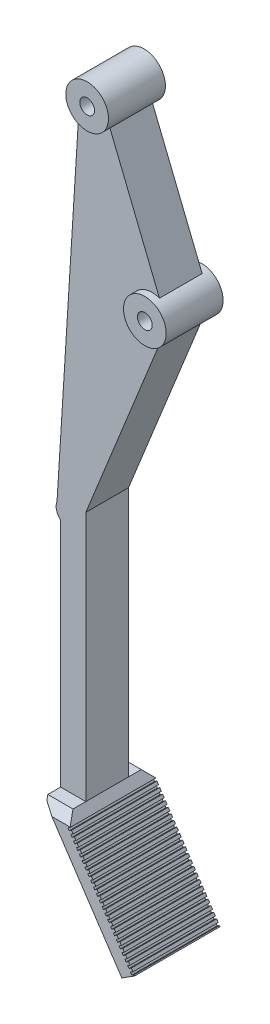
SolidWorks part; units mm, degrees
ref_plane "Front Plane" through (0, 0, 0) normal (0, 0, 1) x (1, 0, 0)
ref_plane "Top Plane" through (0, 0, 0) normal (0, 1, 0) x (1, 0, 0)
ref_plane "Right Plane" through (0, 0, 0) normal (1, 0, 0) x (0, 0, -1)
other "Configuration Table"
sketch "Sketch1" plane through (0, 0, 0) normal (0, 0, 1) x (1, 0, 0)
  circle A0 centre (0, 0) radius 7.5
  dimension "D1" = 15
extrude "Boss-Extrude1" add sketch "Sketch1" along normal mid plane 20
sketch "Sketch2" plane through (0, 0, 0) normal (0, 0, 1) x (1, 0, 0)
  line L0 (0, 0) -> (0, -45.3837) construction
  line L1 (5.5028, -5.096) -> (24.9744, -53.29)
  line L2 (-5.395, -5.2099) -> (15.5663, -57.0911)
  circle A0 centre (0, 0) radius 7.5 construction
  arc A1 (-5.395, -5.2099) -> (5.5028, -5.096) centre (0, 0) ccw
  arc A2 (24.9744, -53.29) -> (15.5663, -57.0911) centre (20.2704, -55.1906) cw
  dimension "D1" = 22
extrude "Boss-Extrude2" add sketch "Sketch2" along normal mid plane 15
sketch "Sketch3" plane through (0, 0, 10) normal (0, 0, 1) x (1, 0, 0)
  circle A0 centre (0, 0) radius 2.6
  dimension "D1" = 5.2
extrude "Cut-Extrude1" cut sketch "Sketch3" against normal through all
sketch "Sketch5" plane through (0, 0, 0) normal (0, 0, 1) x (1, 0, 0)
  line L0 (15.5663, -57.0911) -> (-13.0808, -127.9952)
  line L1 (24.9442, -57.1644) -> (-4.9935, -131.2627)
  line L2 (20.2704, -55.1906) -> (20.2704, -167.243) construction
  arc A0 (15.5663, -57.0911) -> (24.9744, -53.29) centre (20.2704, -55.1906) ccw construction
  arc A1 (15.5663, -57.0911) -> (24.9442, -57.1644) centre (20.2704, -55.1906) ccw
  arc A2 (-13.0808, -127.9952) -> (-4.9935, -131.2627) centre (-9.0371, -129.6289) ccw
  dimension "D1" = 22
  dimension "D2" = 80
extrude "Boss-Extrude3" add sketch "Sketch5" along normal mid plane 15
sketch "Sketch6" plane through (0, 0, 0) normal (0, 0, 1) x (1, 0, 0)
  circle A0 centre (20.2704, -55.1906) radius 7.5
  dimension "D1" = 15
extrude "Boss-Extrude4" add sketch "Sketch6" along normal mid plane 20
sketch "Sketch7" plane through (0, 0, 10) normal (0, 0, 1) x (1, 0, 0)
  circle A0 centre (20.2704, -55.1906) radius 2.6
  dimension "D1" = 5.2
extrude "Cut-Extrude2" cut sketch "Sketch7" against normal through all
sketch "Sketch11" plane through (0, 0, 0) normal (0, 0, 1) x (1, 0, 0)
  line L0 (-5.395, -5.2099) -> (-13.0808, -127.9952)
  line L1 (-5.395, -5.2099) -> (13.4972, -51.9698)
  line L2 (14.4321, -59.8985) -> (-13.0808, -127.9952)
  line L3 (14.4321, -59.8985) -> (-13.0808, -127.9952) construction
  arc A1 (13.4972, -51.9698) -> (14.4321, -59.8985) centre (20.2704, -55.1906) ccw
extrude "Boss-Extrude8" add sketch "Sketch11" along normal mid plane 15
sketch "Sketch16" plane through (0, 0, 0) normal (0, 0, 1) x (1, 0, 0)
  line L0 (-4.9935, -131.2627) -> (22.9045, -62.2128) construction
  line L1 (-11.8087, -126.2616) -> (-2.9729, -126.2616)
  line L2 (-11.8087, -126.2616) -> (-11.8087, -214.2616)
  line L3 (-11.8087, -214.2616) -> (-2.9729, -214.2616)
  line L4 (-2.9729, -126.2616) -> (-2.9729, -214.2616)
  arc A0 (-13.0808, -127.9952) -> (-4.9935, -131.2627) centre (-9.0371, -129.6289) ccw construction
  dimension "D1" = 88
extrude "Boss-Extrude9" add sketch "Sketch16" along normal mid plane 15
sketch "Sketch17" plane through (0, 0, 0) normal (0, 0, -1) x (-1, 0, 0)
  line L3 (11.8087, -214.2616) -> (2.9729, -214.2616)
  line L4 (7.3908, -214.2616) -> (7.3908, -121.3362) construction
  line L5 (-21.6957, -251.2326) -> (2.9729, -214.2616)
  line L6 (-15.4953, -255.1822) -> (-21.6957, -251.2326)
  line L7 (11.8087, -214.2616) -> (-15.4953, -255.1822)
  line L8 (11.8087, -214.2616) -> (2.9729, -214.2616) construction
  line L9 (2.9729, -214.2616) -> (2.9729, -126.2616) construction
  line L10 (11.8087, -132.9962) -> (11.8087, -214.2616) construction
extrude "Boss-Extrude10" add sketch "Sketch17" along normal mid plane 30 contours L3 L5 L6 L7
chamfer "Chamfer1" distance 3 angle 45 2 edges at (-7.3908, -214.2616, 15) (-7.3908, -214.2616, -15)
chamfer "Chamfer2" distance 2 angle 45 2 edges at (2.8442, -236.2219, 15) (2.8442, -236.2219, -15)
sketch "Sketch18" plane through (0, 0, 15) normal (0, 0, 1) x (1, 0, 0)
  line L0 (-0.9223, -217.335) -> (-0.4782, -218.0004)
  line L1 (21.6957, -251.2326) -> (-0.9712, -217.2616) construction
  line L2 (-0.4782, -218.0004) -> (-1.3101, -218.5555)
  line L3 (-1.3101, -218.5555) -> (-1.7541, -217.89)
  line L4 (-1.7541, -217.89) -> (-0.9223, -217.335)
  line L97 (-0.755, -219.3873) -> (0.0768, -218.8323)
  line L98 (0.0768, -218.8323) -> (0.5208, -219.4977)
  line L99 (0.5208, -219.4977) -> (-0.311, -220.0528)
  line L100 (-0.311, -220.0528) -> (-0.755, -219.3873)
  line L101 (0.244, -220.8846) -> (1.0759, -220.3296)
  line L102 (1.0759, -220.3296) -> (1.5199, -220.995)
  line L103 (1.5199, -220.995) -> (0.6881, -221.55)
  line L104 (0.6881, -221.55) -> (0.244, -220.8846)
  line L105 (1.2431, -222.3819) -> (2.0749, -221.8268)
  line L106 (2.0749, -221.8268) -> (2.5189, -222.4923)
  line L107 (2.5189, -222.4923) -> (1.6871, -223.0473)
  line L108 (1.6871, -223.0473) -> (1.2431, -222.3819)
  line L109 (2.2421, -223.8792) -> (3.074, -223.3241)
  line L110 (3.074, -223.3241) -> (3.518, -223.9896)
  line L111 (3.518, -223.9896) -> (2.6862, -224.5446)
  line L112 (2.6862, -224.5446) -> (2.2421, -223.8792)
  line L113 (3.2412, -225.3765) -> (4.073, -224.8214)
  line L114 (4.073, -224.8214) -> (4.5171, -225.4869)
  line L115 (4.5171, -225.4869) -> (3.6852, -226.0419)
  line L116 (3.6852, -226.0419) -> (3.2412, -225.3765)
  line L117 (4.2403, -226.8737) -> (5.0721, -226.3187)
  line L118 (5.0721, -226.3187) -> (5.5161, -226.9842)
  line L119 (5.5161, -226.9842) -> (4.6843, -227.5392)
  line L120 (4.6843, -227.5392) -> (4.2403, -226.8737)
  line L121 (5.2393, -228.371) -> (6.0711, -227.816)
  line L122 (6.0711, -227.816) -> (6.5152, -228.4815)
  line L123 (6.5152, -228.4815) -> (5.6833, -229.0365)
  line L124 (5.6833, -229.0365) -> (5.2393, -228.371)
  line L125 (6.2384, -229.8683) -> (7.0702, -229.3133)
  line L126 (7.0702, -229.3133) -> (7.5142, -229.9788)
  line L127 (7.5142, -229.9788) -> (6.6824, -230.5338)
  line L128 (6.6824, -230.5338) -> (6.2384, -229.8683)
  line L129 (7.2374, -231.3656) -> (8.0693, -230.8106)
  line L130 (8.0693, -230.8106) -> (8.5133, -231.4761)
  line L131 (8.5133, -231.4761) -> (7.6815, -232.0311)
  line L132 (7.6815, -232.0311) -> (7.2374, -231.3656)
  line L133 (8.2365, -232.8629) -> (9.0683, -232.3079)
  line L134 (9.0683, -232.3079) -> (9.5124, -232.9733)
  line L135 (9.5124, -232.9733) -> (8.6805, -233.5284)
  line L136 (8.6805, -233.5284) -> (8.2365, -232.8629)
  line L137 (9.2356, -234.3602) -> (10.0674, -233.8052)
  line L138 (10.0674, -233.8052) -> (10.5114, -234.4706)
  line L139 (10.5114, -234.4706) -> (9.6796, -235.0257)
  line L140 (9.6796, -235.0257) -> (9.2356, -234.3602)
  line L141 (10.2346, -235.8575) -> (11.0664, -235.3025)
  line L142 (11.0664, -235.3025) -> (11.5105, -235.9679)
  line L143 (11.5105, -235.9679) -> (10.6786, -236.523)
  line L144 (10.6786, -236.523) -> (10.2346, -235.8575)
  line L145 (11.2337, -237.3548) -> (12.0655, -236.7998)
  line L146 (12.0655, -236.7998) -> (12.5095, -237.4652)
  line L147 (12.5095, -237.4652) -> (11.6777, -238.0203)
  line L148 (11.6777, -238.0203) -> (11.2337, -237.3548)
  line L149 (12.2327, -238.8521) -> (13.0646, -238.297)
  line L150 (13.0646, -238.297) -> (13.5086, -238.9625)
  line L151 (13.5086, -238.9625) -> (12.6768, -239.5175)
  line L152 (12.6768, -239.5175) -> (12.2327, -238.8521)
  line L153 (13.2318, -240.3494) -> (14.0636, -239.7943)
  line L154 (14.0636, -239.7943) -> (14.5076, -240.4598)
  line L155 (14.5076, -240.4598) -> (13.6758, -241.0148)
  line L156 (13.6758, -241.0148) -> (13.2318, -240.3494)
  line L157 (14.2308, -241.8467) -> (15.0627, -241.2916)
  line L158 (15.0627, -241.2916) -> (15.5067, -241.9571)
  line L159 (15.5067, -241.9571) -> (14.6749, -242.5121)
  line L160 (14.6749, -242.5121) -> (14.2308, -241.8467)
  line L161 (15.2299, -243.344) -> (16.0617, -242.7889)
  line L162 (16.0617, -242.7889) -> (16.5058, -243.4544)
  line L163 (16.5058, -243.4544) -> (15.6739, -244.0094)
  line L164 (15.6739, -244.0094) -> (15.2299, -243.344)
  line L165 (16.229, -244.8412) -> (17.0608, -244.2862)
  line L166 (17.0608, -244.2862) -> (17.5048, -244.9517)
  line L167 (17.5048, -244.9517) -> (16.673, -245.5067)
  line L168 (16.673, -245.5067) -> (16.229, -244.8412)
  line L169 (17.228, -246.3385) -> (18.0599, -245.7835)
  line L170 (18.0599, -245.7835) -> (18.5039, -246.449)
  line L171 (18.5039, -246.449) -> (17.672, -247.004)
  line L172 (17.672, -247.004) -> (17.228, -246.3385)
  line L173 (18.2271, -247.8358) -> (19.0589, -247.2808)
  line L174 (19.0589, -247.2808) -> (19.5029, -247.9463)
  line L175 (19.5029, -247.9463) -> (18.6711, -248.5013)
  line L176 (18.6711, -248.5013) -> (18.2271, -247.8358)
  line L177 (19.2261, -249.3331) -> (20.058, -248.7781)
  line L178 (20.058, -248.7781) -> (20.502, -249.4436)
  line L179 (20.502, -249.4436) -> (19.6702, -249.9986)
  line L180 (19.6702, -249.9986) -> (19.2261, -249.3331)
  line L181 (20.2252, -250.8304) -> (21.057, -250.2754)
  line L182 (21.057, -250.2754) -> (21.5011, -250.9408)
  line L183 (21.5011, -250.9408) -> (20.6692, -251.4959)
  line L184 (20.6692, -251.4959) -> (20.2252, -250.8304)
  line L185 (21.2243, -252.3277) -> (22.0561, -251.7727)
  line L186 (22.0561, -251.7727) -> (22.5001, -252.4381)
  line L187 (22.5001, -252.4381) -> (21.6683, -252.9932)
  line L188 (21.6683, -252.9932) -> (21.2243, -252.3277)
  dimension "D1" = 0.8
  dimension "D2" = 1
  dimension "D4" = 1
  dimension "D3" = 24
extrude "Cut-Extrude3" cut sketch "Sketch18" against normal through all
